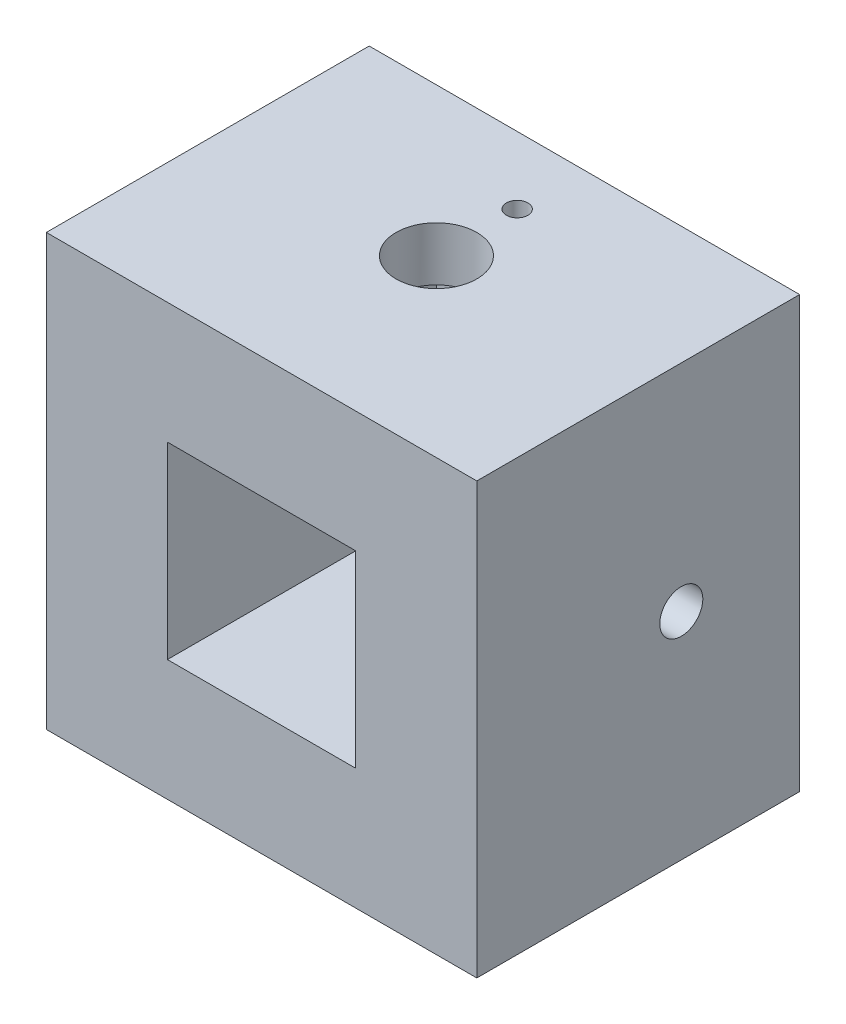
from build123d import *

# Parameters (mm, degrees)
BOSS_EXTRUDE1_START     = 10
SKETCH1_W               = 80
SKETCH1_H               = 80
BOSS_EXTRUDE1_DEPTH     = 50
SKETCH2_W               = 35
SKETCH2_H               = 35
CUT_EXTRUDE1_DEPTH      = 45
SKETCH3_W               = 55
SKETCH3_H               = 55
CUT_EXTRUDE2_DEPTH      = 5
SKETCH4_W               = 15
SKETCH4_H               = 15
CUT_EXTRUDE3_DEPTH      = 156
BOSS_EXTRUDE2_DEPTH     = 10
BOSS_EXTRUDE3_START     = -10
BOSS_EXTRUDE3_DEPTH     = 10
SKETCH9_R               = 4
CUT_EXTRUDE6_DEPTH      = 99
SKETCH13_W              = 35
SKETCH13_H              = 35
CUT_EXTRUDE7_DEPTH      = 200
CUT_EXTRUDE8_DEPTH      = 160.525859973
CUT_EXTRUDE8_DEPTH_BACK = 43
SKETCH14_R              = 2
SKETCH15_W              = 80
SKETCH15_H              = 80
SKETCH15_W_2            = 55
SKETCH15_H_2            = 55
BOSS_EXTRUDE4_DEPTH     = 10


with BuildPart() as part:
    # Sketch1 → Boss-Extrude1 (new body)
    with BuildSketch(Plane.XY.offset(BOSS_EXTRUDE1_START)):
        with Locations((-91.5, -21.5)):
            Rectangle(SKETCH1_W, SKETCH1_H)
    extrude(amount=BOSS_EXTRUDE1_DEPTH)

    # Sketch2 → Cut-Extrude1 (cut)
    with BuildSketch(Plane(origin=(0, 0, 10), x_dir=(-1, 0, 0), z_dir=(0, 0, -1))):
        with Locations((91.5, -21.5)):
            Rectangle(SKETCH2_W, SKETCH2_H)
    extrude(amount=-CUT_EXTRUDE1_DEPTH, mode=Mode.SUBTRACT)

    # Sketch3 → Cut-Extrude2 (cut)
    with BuildSketch(Plane(origin=(0, 0, 10), x_dir=(-1, 0, 0), z_dir=(0, 0, -1))):
        with Locations((91.5, -21.5)):
            Rectangle(SKETCH3_W, SKETCH3_H)
    extrude(amount=-CUT_EXTRUDE2_DEPTH, mode=Mode.SUBTRACT)

    # Sketch4 → Cut-Extrude3 (cut)
    with BuildSketch(Plane(origin=(0, -61.5, 0), x_dir=(-1, 0, 0), z_dir=(0, -1, 0))):
        with Locations((91.5, -27.5)):
            Rectangle(SKETCH4_W, SKETCH4_H)
    extrude(amount=-CUT_EXTRUDE3_DEPTH, mode=Mode.SUBTRACT)

    # Sketch5 → Boss-Extrude2 (add)
    with BuildSketch(Plane.XZ.offset(61.5)):
        with BuildLine():
            Line((-99, 27.5), (-99, 20))
            Line((-99, 20), (-91.499999963, 20))
            ThreePointArc((-91.499999963, 20), (-96.803300846, 22.196699128), (-99, 27.5))
        make_face()
        with BuildLine():
            ThreePointArc((-84, 27.5), (-86.196699128, 22.196699154), (-91.499999963, 20))
            Line((-91.499999963, 20), (-84, 20))
            Line((-84, 20), (-84, 27.5))
        make_face()
        with BuildLine():
            ThreePointArc((-91.5, 35), (-86.196699141, 32.803300859), (-84, 27.5))
            Line((-84, 27.5), (-84, 35))
            Line((-84, 35), (-91.5, 35))
        make_face()
        with BuildLine():
            Line((-99, 35), (-99, 27.5))
            ThreePointArc((-99, 27.5), (-96.803300859, 32.803300859), (-91.5, 35))
            Line((-91.5, 35), (-99, 35))
        make_face()
    extrude(amount=-BOSS_EXTRUDE2_DEPTH)

    # Sketch6 → Boss-Extrude3 (add)
    with BuildSketch(Plane(origin=(0, 18.5, 0), x_dir=(1, 0, 0), z_dir=(0, 1, 0)).offset(BOSS_EXTRUDE3_START)):
        with BuildLine():
            Line((-84, -27.5), (-84, -20))
            Line((-84, -20), (-91.5, -20))
            ThreePointArc((-91.5, -20), (-86.196699141, -22.196699141), (-84, -27.5))
        make_face()
        with BuildLine():
            ThreePointArc((-99, -27.5), (-96.803300859, -22.196699141), (-91.5, -20))
            Line((-91.5, -20), (-99, -20))
            Line((-99, -20), (-99, -27.5))
        make_face()
        with BuildLine():
            ThreePointArc((-91.5, -35), (-96.803300859, -32.803300859), (-99, -27.5))
            Line((-99, -27.5), (-99, -35))
            Line((-99, -35), (-91.5, -35))
        make_face()
        with BuildLine():
            Line((-84, -35), (-84, -27.5))
            ThreePointArc((-84, -27.5), (-86.196699141, -32.803300859), (-91.5, -35))
            Line((-91.5, -35), (-84, -35))
        make_face()
    extrude(amount=BOSS_EXTRUDE3_DEPTH)

    # Sketch9 → Cut-Extrude6 (cut)
    with BuildSketch(Plane.ZY.offset(131.5)):
        with Locations((22, -21.5)):
            Circle(SKETCH9_R)
    extrude(amount=-CUT_EXTRUDE6_DEPTH, mode=Mode.SUBTRACT)

    # Sketch13 → Cut-Extrude7 (cut)
    with BuildSketch(Plane(origin=(0, 0, 55), x_dir=(-1, 0, 0), z_dir=(0, 0, -1))):
        with Locations((91.5, -21.5)):
            Rectangle(SKETCH13_W, SKETCH13_H)
    extrude(amount=-CUT_EXTRUDE7_DEPTH, mode=Mode.SUBTRACT)

    # Sketch14 → Cut-Extrude8 (cut, two sides: drawn at the far end of the back side and taken through both)
    with BuildSketch(Plane(origin=(0, -49, 0), x_dir=(1, 0, 0), z_dir=(0, 1, 0)).offset(-CUT_EXTRUDE8_DEPTH_BACK)):
        with Locations(Location((-91.5, -12.5, 0), (0, 0, 270))):
            Circle(SKETCH14_R)
    extrude(amount=CUT_EXTRUDE8_DEPTH + CUT_EXTRUDE8_DEPTH_BACK, mode=Mode.SUBTRACT)

    # Sketch15 → Boss-Extrude4 (add)
    with BuildSketch(Plane(origin=(0, 0, 10), x_dir=(-1, 0, 0), z_dir=(0, 0, -1))):
        with Locations((91.5, -21.5)):
            Rectangle(SKETCH15_W, SKETCH15_H)
        with Locations((91.5, -21.5)):
            Rectangle(SKETCH15_W_2, SKETCH15_H_2, mode=Mode.SUBTRACT)
    extrude(amount=BOSS_EXTRUDE4_DEPTH)


solid = part.part
